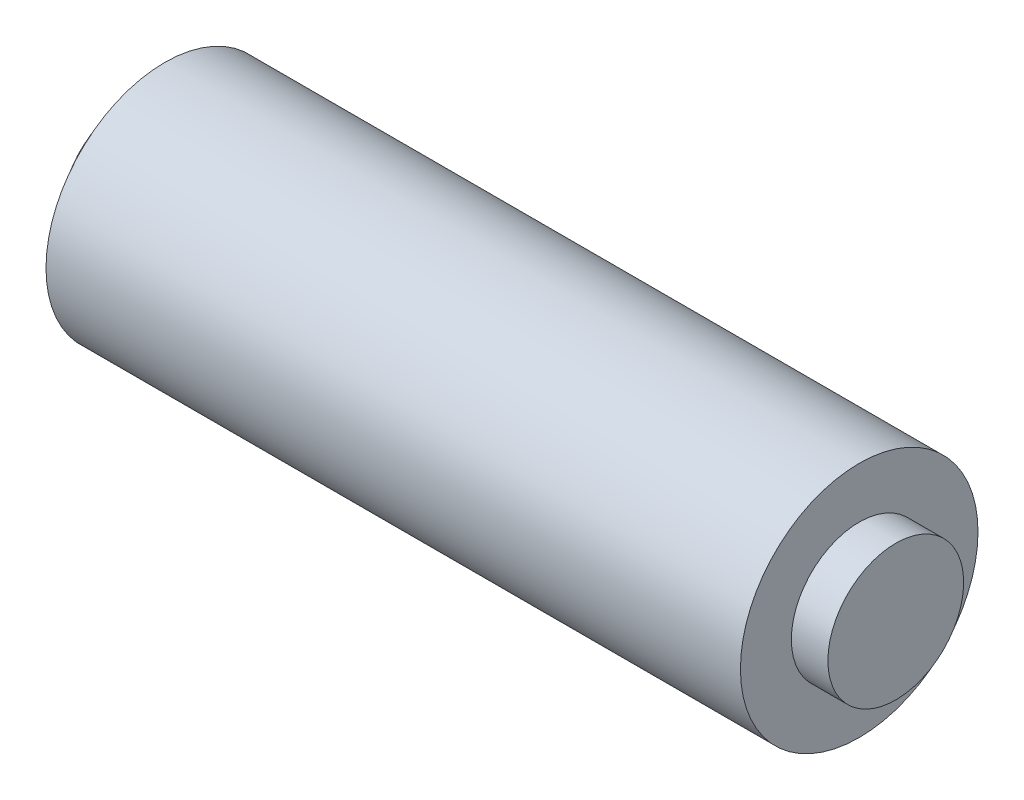
from build123d import *


with BuildPart() as part:
    # 草图1 → 旋转1 (revolve)
    with BuildSketch(Plane.XY, mode=Mode.PRIVATE) as revolve_1_sk:
        Polygon((-21, 0), (-21, 3.714285714), (-19, 3.714285714), (-19, 6.5), (19, 6.5), (19, 3.714285714), (21, 3.714285714), (21, 0), align=None)
    revolve(revolve_1_sk.sketch.rotate(Axis((21, 0, 0), (-1, 0, 0)), 270), axis=Axis((21, 0, 0), (-1, 0, 0)))


solid = part.part
